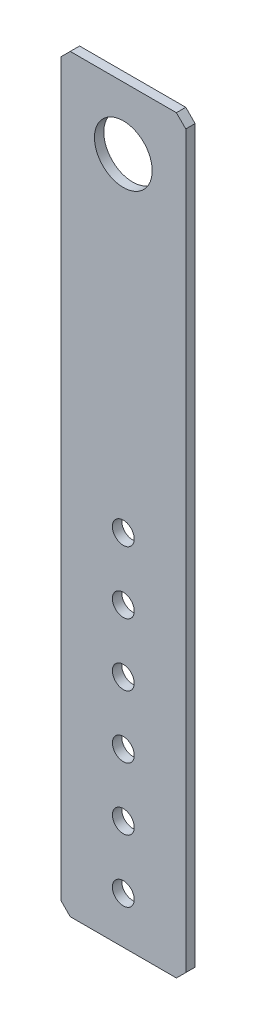
SolidWorks part; units mm, degrees
ref_plane "Front Plane" through (0, 0, 0) normal (0, 0, 1) x (1, 0, 0)
ref_plane "Top Plane" through (0, 0, 0) normal (0, 1, 0) x (1, 0, 0)
ref_plane "Right Plane" through (0, 0, 0) normal (1, 0, 0) x (0, 0, -1)
sketch "Sketch1" plane through (0, 0, 0) normal (0, 0, 1) x (1, 0, 0)
  line L0 (-20, 117) -> (-17, 120)
  line L1 (17, -120) -> (-17, -120)
  line L2 (20, -117) -> (20, 117)
  line L3 (17, 120) -> (-17, 120)
  line L4 (-20, -117) -> (-20, 117)
  line L5 (20, -120) -> (-20, 120) construction
  line L6 (20, 120) -> (-20, -120) construction
  line L7 (20, 117) -> (17, 120)
  line L8 (-17, -120) -> (-20, -117)
  line L9 (17, -120) -> (20, -117)
  line L10 (0, 120) -> (0, -120) construction
  circle A0 centre (0, 100) radius 9.25
  circle A1 centre (0, -105) radius 3.5
  circle A2 centre (0, -85) radius 3.5
  circle A3 centre (0, -65) radius 3.5
  circle A4 centre (0, -45) radius 3.5
  circle A5 centre (0, -25) radius 3.5
  circle A6 centre (0, -5) radius 3.5
  point P0 (0, 0)
  dimension "D3" = 18.5
  dimension "D4" = 220
  dimension "D9" = 7
  dimension "D10" = 15
  dimension "D1" = 40
  dimension "D2" = 240
  dimension "D11" = 6
extrude "Boss-Extrude1" add sketch "Sketch1" along normal mid plane 3
